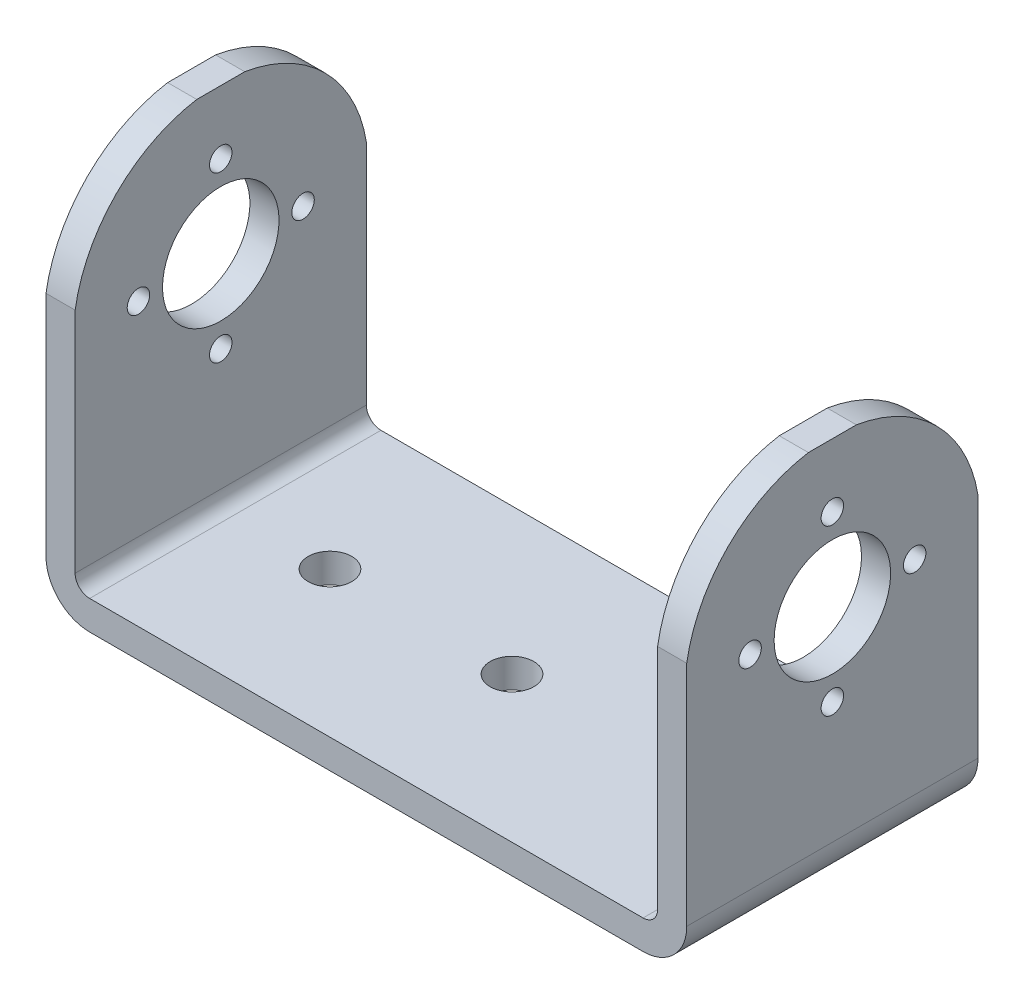
SolidWorks part; units mm, degrees
ref_plane "Front Plane" through (0, 0, 0) normal (0, 0, 1) x (1, 0, 0)
ref_plane "Top Plane" through (0, 0, 0) normal (0, 1, 0) x (1, 0, 0)
ref_plane "Right Plane" through (0, 0, 0) normal (1, 0, 0) x (0, 0, -1)
other "Configuration Table"
sketch "Sketch1" plane through (0, 0, 0) normal (0, 0, 1) x (1, 0, 0)
  line L0 (0, 25) -> (0, 1)
  line L1 (1, 0) -> (39, 0)
  line L2 (40, 1) -> (40, 25)
  line L3 (-2, 25) -> (-2, 1)
  line L4 (1, -2) -> (39, -2)
  line L5 (42, 1) -> (42, 25)
  line L6 (-2, 25) -> (0, 25)
  line L7 (40, 25) -> (42, 25)
  line L8 (0, 0) -> (40, 0) construction
  line L9 (40, 0) -> (40, 25) construction
  line L10 (0, 25) -> (0, 0) construction
  line L11 (-2, -2) -> (42, -2) construction
  line L12 (42, -2) -> (42, 25) construction
  line L13 (-2, 25) -> (-2, -2) construction
  arc A0 (39, 0) -> (40, 1) centre (39, 1) ccw
  arc A1 (0, 1) -> (1, 0) centre (1, 1) ccw
  arc A2 (39, -2) -> (42, 1) centre (39, 1) ccw
  arc A3 (-2, 1) -> (1, -2) centre (1, 1) ccw
  point P12 (40, 0)
  dimension "D4" = 1
  dimension "D1" = 3
  dimension "D3" = 2
extrude "Boss-Extrude1" add sketch "Sketch1" along normal blind 20
sketch "Sketch2" plane through (-2, 0, 0) normal (-1, 0, 0) x (0, 0, 1)
  line L0 (20, 25) -> (0, 25) construction
  line L1 (-0.1348, 15) -> (-9.48, 25.1348)
  line L2 (-9.48, 25.1348) -> (9.1999, 33.7111)
  line L3 (9.1999, 33.7111) -> (31.2192, 26.9279)
  line L4 (31.2192, 26.9279) -> (20.1348, 15)
  circle A0 centre (10, 15) radius 4
  arc A1 (20.1348, 15) -> (-0.1348, 15) centre (10, 15) ccw
  circle A2 centre (10, 20.6512) radius 0.7713
  circle A3 centre (15.6512, 15) radius 0.7713
  circle A4 centre (10, 9.3488) radius 0.7713
  circle A5 centre (4.3488, 15) radius 0.7713
  dimension "D1" = 8
  dimension "D2" = 10
  dimension "D3" = 4
extrude "Cut-Extrude1" cut sketch "Sketch2" against normal through all
sketch "Sketch3" plane through (0, 0, 0) normal (0, 1, 0) x (1, 0, 0)
  line L0 (1, -10) -> (39, -10) construction
  line L1 (1, -20) -> (1, 0) construction
  line L2 (39, -20) -> (39, 0) construction
  line L3 (7.5, -10) -> (7.5, -3.1778) construction
  line L4 (32.5, -10) -> (32.5, -3.1778) construction
  line L5 (20, -10) -> (20, -4.8337) construction
  circle A0 centre (7.5, -10) radius 1.5
  circle A1 centre (20, -10) radius 1.5
  circle A2 centre (32.5, -10) radius 1.5
  dimension "D3" = 3
  dimension "D4" = 3
  dimension "D5" = 3
  dimension "D1" = 25
  dimension "D2" = 12.5
extrude "Cut-Extrude2" cut sketch "Sketch3" against normal through all
